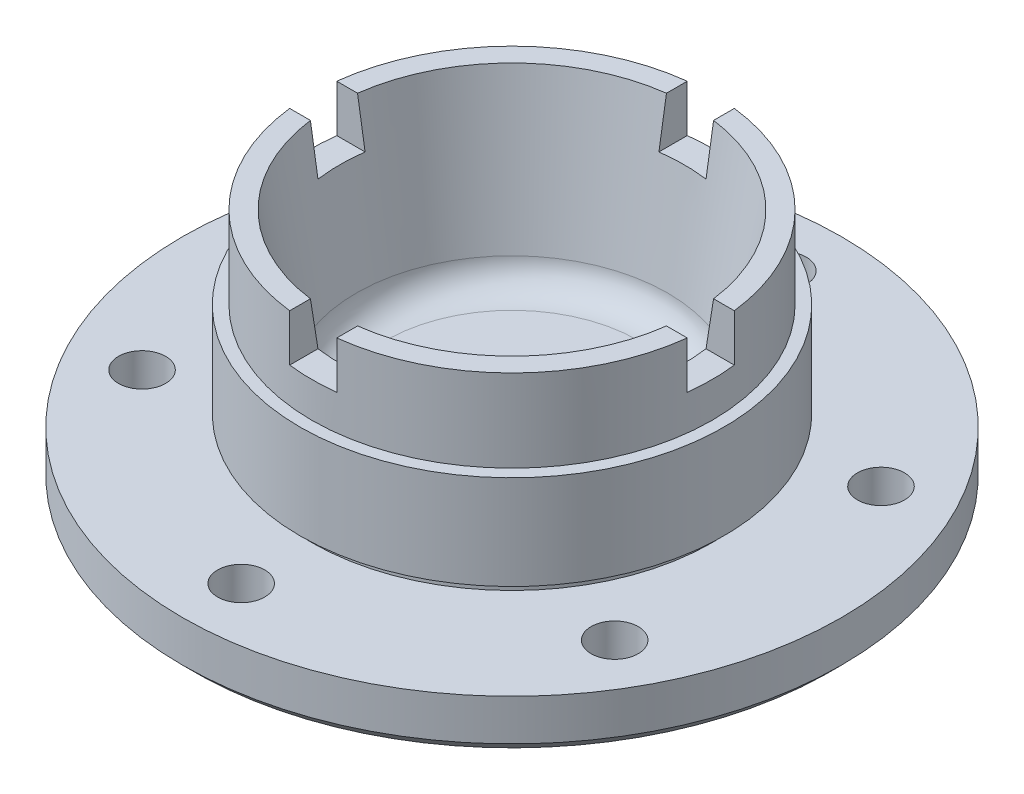
SolidWorks part; units mm, degrees
ref_plane "Front" through (0, 0, 0) normal (0, 0, 1) x (1, 0, 0)
ref_plane "Top" through (0, 0, 0) normal (0, 1, 0) x (1, 0, 0)
ref_plane "Right" through (0, 0, 0) normal (1, 0, 0) x (0, 0, -1)
sketch "Sketch1" plane through (0, 0, 0) normal (0, 0, 1) x (1, 0, 0)
  line L0 (32, 0) -> (54, 0)
  line L1 (56, 2) -> (56, 9)
  line L2 (56, 9) -> (36, 9)
  line L3 (36, 11) -> (36, 27)
  line L4 (36, 27) -> (34, 27)
  line L5 (34, 27) -> (34, 41)
  line L6 (34, 41) -> (30.5, 41)
  line L7 (0, 11) -> (21.4751, 11)
  line L8 (0, 2) -> (0, 11)
  line L10 (0, 2) -> (31, 2)
  line L11 (54, 0) -> (56, 2)
  line L12 (31, 2) -> (32, 0)
  line L13 (36, 9) -> (34, 9)
  line L14 (34, 9) -> (34, 11)
  line L15 (34, 11) -> (36, 11)
  line L17 (26.4502, 15.5025) -> (30.5, 41)
  arc A0 (26.4502, 15.5025) -> (21.4751, 11) centre (21.4751, 16) cw
  point P1 (56, 0)
  dimension "D9" = 5
  dimension "D2" = 9
  dimension "D3" = 20
  dimension "D4" = 18
  dimension "D5" = 2
  dimension "D6" = 14
  dimension "D8" = 11
  dimension "D10" = 2
  dimension "D11" = 31
  dimension "D12" = 2
  dimension "D13" = 2
revolve "Revolve1" add sketch "Sketch1" angle 360 about L8
sketch "Sketch2" plane through (0, 41, 0) normal (0, 1, 0) x (1, 0, 0)
  line L0 (37.2623, 4) -> (17.2623, 4)
  line L1 (-4, 37.2623) -> (4, 37.2623)
  line L2 (-4, 37.2623) -> (-4, 17.2623)
  line L3 (-4, 17.2623) -> (4, 17.2623)
  line L4 (4, 37.2623) -> (4, 17.2623)
  line L5 (37.2623, 4) -> (37.2623, -4)
  line L6 (37.2623, -4) -> (17.2623, -4)
  line L7 (17.2623, 4) -> (17.2623, -4)
  line L8 (4, -37.2623) -> (4, -17.2623)
  line L9 (4, -37.2623) -> (-4, -37.2623)
  line L10 (-4, -37.2623) -> (-4, -17.2623)
  line L11 (4, -17.2623) -> (-4, -17.2623)
  line L12 (-37.2623, -4) -> (-17.2623, -4)
  line L13 (-37.2623, -4) -> (-37.2623, 4)
  line L14 (-37.2623, 4) -> (-17.2623, 4)
  line L15 (-17.2623, -4) -> (-17.2623, 4)
  point P20 (0, 0)
  dimension "D1" = 8
  dimension "D2" = 20
  dimension "D3" = 4
  dimension "D4" = 4
extrude "Cut-Extrude1" cut sketch "Sketch2" against normal blind 8
sketch "Sketch3" plane through (0, 41, 0) normal (0, 1, 0) x (1, 0, 0)
  line L0 (0, 0) -> (53.9742, 0) construction
  line L1 (0, 0) -> (0, 60.1002) construction
  line L2 (0, 0) -> (56.153, 32.42) construction
  line L3 (0, 0) -> (-58.8967, 34.004) construction
  circle A1 centre (0, 46) radius 4
  circle A2 centre (40.0566, 22.6156) radius 4
  circle A3 centre (-39.8372, 23) radius 4
  circle A4 centre (-39.8372, -23) radius 4
  circle A5 centre (0, -46) radius 4
  circle A6 centre (40.0566, -22.6156) radius 4
  dimension "D4" = 8
  dimension "D5" = 8
  dimension "D6" = 8
  dimension "D1" = 60
  dimension "D2" = 60
extrude "Cut-Extrude2" cut sketch "Sketch3" against normal blind 100
scale "Scale 1" bodies to scale 103 scale about centroid uniform scaling yes scale factor 1.875
